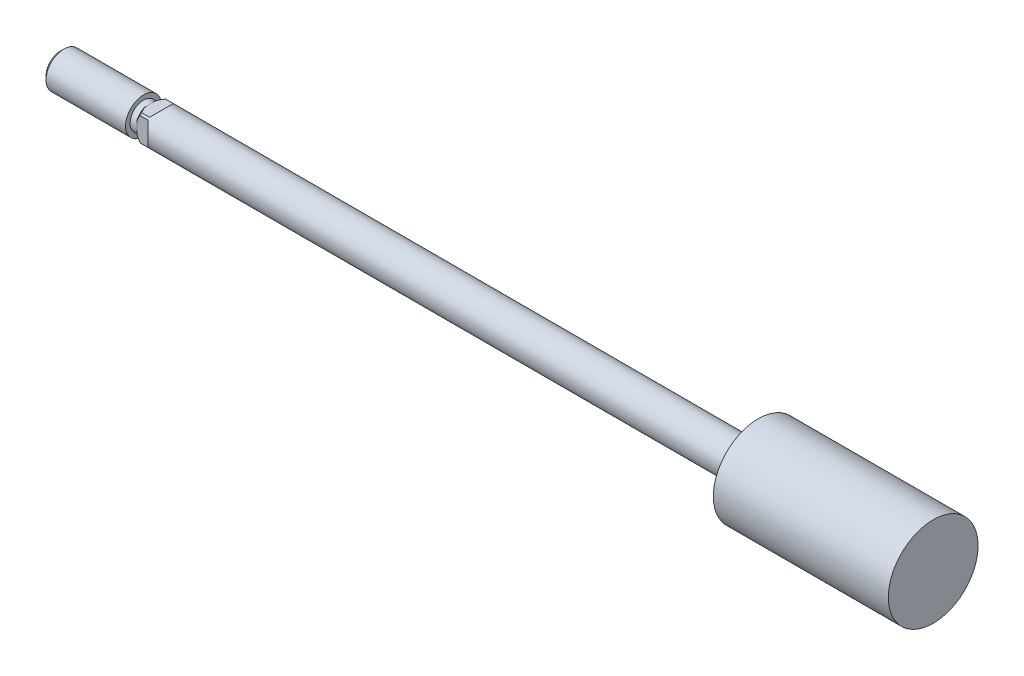
from build123d import *

# Parameters (mm, degrees)
CUT_EXTRUDE_1_DEPTH      = 4
CUT_EXTRUDE_1_DEPTH_BACK = 4
CUT_EXTRUDE_2_DEPTH      = 4
CUT_EXTRUDE_2_DEPTH_BACK = 4
CUT_EXTRUDE_3_DEPTH      = 4
CUT_EXTRUDE_3_DEPTH_BACK = 4
CUT_EXTRUDE_4_DEPTH      = 4
CUT_EXTRUDE_4_DEPTH_BACK = 4
SCALE_1_SCALE            = 0.5


with BuildPart() as part:
    # 草图1 → 旋转1 (revolve)
    with BuildSketch(Plane.XY, mode=Mode.PRIVATE) as revolve_1_sk:
        Polygon((-40, 0), (-40, 3.233), (-39.233, 4), (-21.5, 4), (-21.5, 3), (-20, 3), (-20, 3.25), (-19.25, 4), (115.5, 4), (115.5, 10), (154.5, 10), (154.5, 0), align=None)
    revolve(revolve_1_sk.sketch.rotate(Axis((154.5, 0, 0), (-1, 0, 0)), 270), axis=Axis((154.5, 0, 0), (-1, 0, 0)))

    # 草图2 → 切除-拉伸1 (cut, two sides: drawn at the far end of the back side and taken through both)
    with BuildSketch(Plane.XY.offset(-CUT_EXTRUDE_1_DEPTH_BACK)):
        Polygon((-20, 3), (-17.5, 3), (-16.5, 4), (-20, 4), align=None)
    extrude(amount=CUT_EXTRUDE_1_DEPTH + CUT_EXTRUDE_1_DEPTH_BACK, mode=Mode.SUBTRACT)

    # 草图3 → 切除-拉伸2 (cut, two sides: drawn at the far end of the back side and taken through both)
    with BuildSketch(Plane.XY.offset(-CUT_EXTRUDE_2_DEPTH_BACK)):
        Polygon((-20, -3), (-20, -4), (-16.5, -4), (-17.5, -3), align=None)
    extrude(amount=CUT_EXTRUDE_2_DEPTH + CUT_EXTRUDE_2_DEPTH_BACK, mode=Mode.SUBTRACT)

    # 草图4 → 切除-拉伸3 (cut, two sides: drawn at the far end of the back side and taken through both)
    with BuildSketch(Plane(origin=(0, 0, 0), x_dir=(1, 0, 0), z_dir=(0, 1, 0)).offset(-CUT_EXTRUDE_3_DEPTH_BACK)):
        Polygon((-20, 3), (-17.5, 3), (-16.5, 4), (-20, 4), align=None)
    extrude(amount=CUT_EXTRUDE_3_DEPTH + CUT_EXTRUDE_3_DEPTH_BACK, mode=Mode.SUBTRACT)

    # 草图5 → 切除-拉伸4 (cut, two sides: drawn at the far end of the back side and taken through both)
    with BuildSketch(Plane(origin=(0, 0, 0), x_dir=(1, 0, 0), z_dir=(0, 1, 0)).offset(-CUT_EXTRUDE_4_DEPTH_BACK)):
        Polygon((-20, -3), (-20, -4), (-16.5, -4), (-17.5, -3), align=None)
    extrude(amount=CUT_EXTRUDE_4_DEPTH + CUT_EXTRUDE_4_DEPTH_BACK, mode=Mode.SUBTRACT)


with BuildPart() as part_1:
    # 缩放比例1: scaled about (97.615985287, 0, 0)
    add(part.part.scale(SCALE_1_SCALE).moved(Location((48.807992644, 0, 0))))


solid = part_1.part
